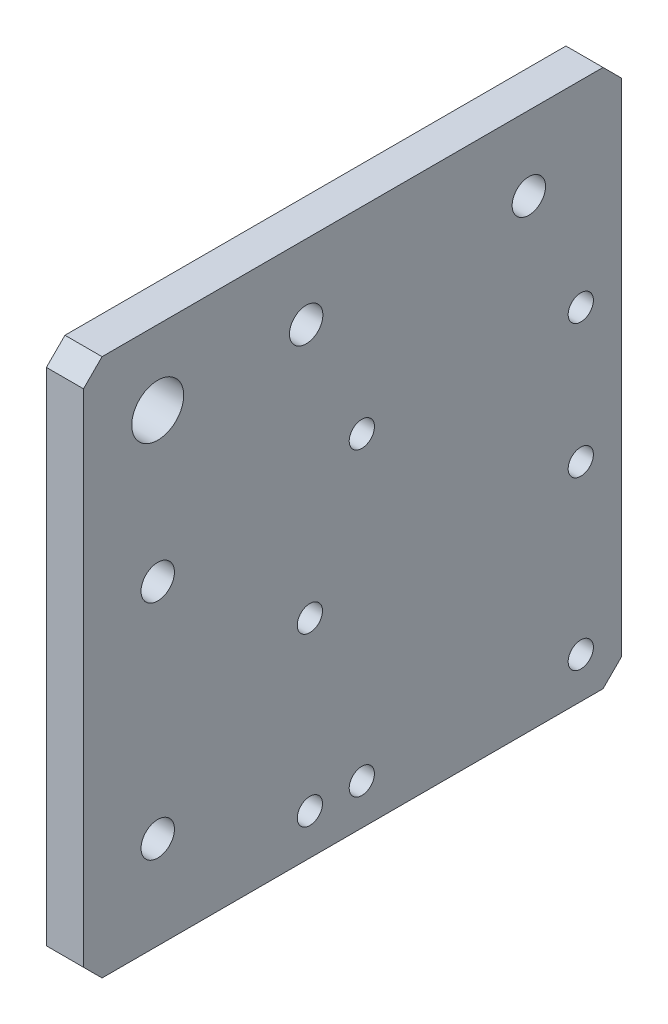
from build123d import *

# Parameters (mm, degrees)
SKETCH_1_W          = 145
SKETCH_1_H          = 145
EXTRUDE_1_DEPTH     = 10
CHAMFER_1_SIZE      = 5
HOLE_WIZARD_M8_1_D  = 6.8
HOLE_WIZARD_M16_1_D = 14
SKETCH_8_R          = 4.5
CUT_EXTRUDE_1_DEPTH = 104.01698889


with BuildPart() as part:
    # 草图1 → 凸台-拉伸1 (new body)
    with BuildSketch(Plane(origin=(0, 0, 0), x_dir=(0, 0, -1), z_dir=(1, 0, 0))):
        Rectangle(SKETCH_1_W, SKETCH_1_H)
    extrude(amount=EXTRUDE_1_DEPTH)

    # 倒角1
    chamfer_1_edges = [part.edges().sort_by_distance(p)[0] for p in [
        (5, -72.5, -72.5),
        (5, -72.5, 72.5),
        (5, 72.5, 72.5),
        (5, 72.5, -72.5),
    ]]
    chamfer(chamfer_1_edges, length=CHAMFER_1_SIZE)

    # M8 螺纹孔1 (through all)
    with Locations(Plane(origin=(10, 0, 0), x_dir=(0, 0, -1), z_dir=(1, 0, 0))):
        with Locations((61.5, -61.5), (2.5, 19.5), (61.5, 19.5), (2.5, -61.5), (-11.5, -61.5), (-11.5, -16.5), (61.5, -16.5)):
            Hole(HOLE_WIZARD_M8_1_D / 2)

    # M16 螺纹孔1 (through all)
    with Locations(Plane(origin=(10, 0, 0), x_dir=(0, 0, -1), z_dir=(1, 0, 0))):
        with Locations((-52.5, 52.5)):
            Hole(HOLE_WIZARD_M16_1_D / 2)

    # 草图8 → 切除-拉伸1 (cut, through all)
    with BuildSketch(Plane(origin=(10, 0, 0), x_dir=(0, 0, -1), z_dir=(1, 0, 0))):
        with Locations((-12.5, 52.5)):
            Circle(SKETCH_8_R)
        with Locations((47.5, 52.5)):
            Circle(SKETCH_8_R)
        with Locations((-52.5, 12.5)):
            Circle(SKETCH_8_R)
        with Locations((-52.5, -47.5)):
            Circle(SKETCH_8_R)
    extrude(amount=-CUT_EXTRUDE_1_DEPTH, mode=Mode.SUBTRACT)


solid = part.part
